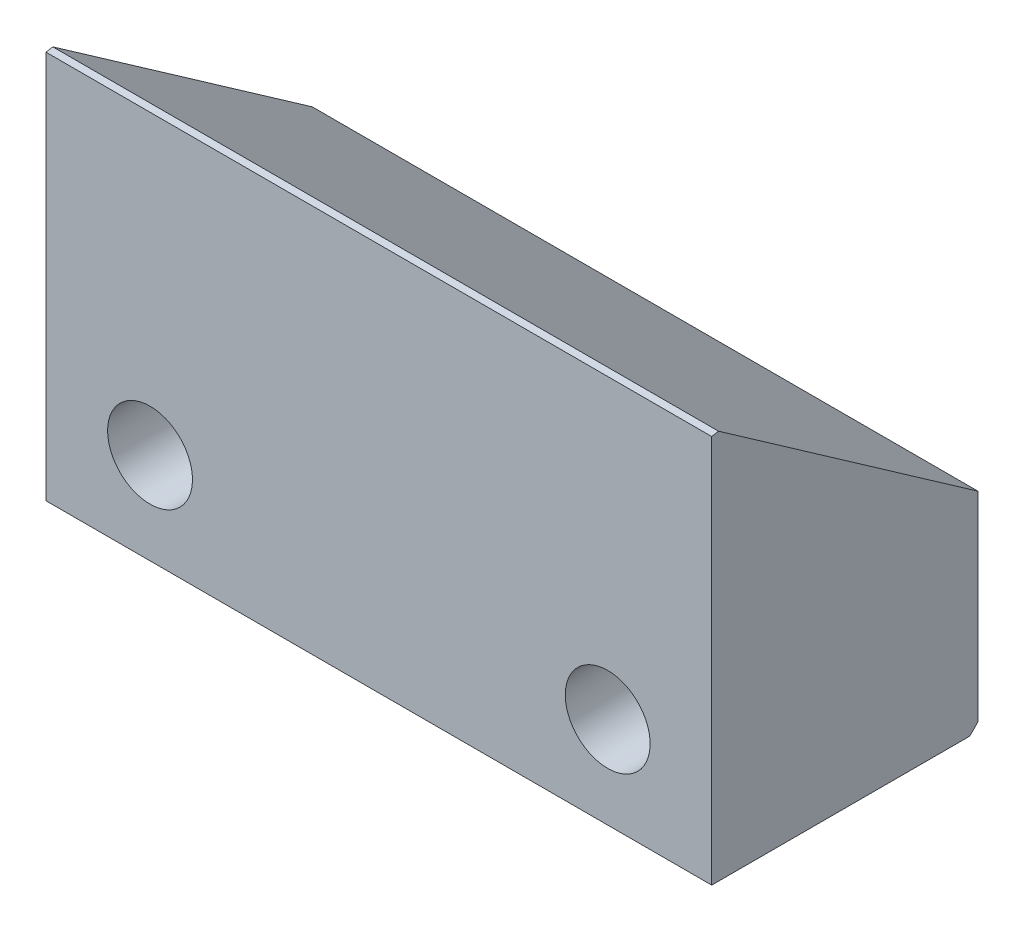
SolidWorks part; units mm, degrees
ref_plane "Front Plane" through (0, 0, 0) normal (0, 0, 1) x (1, 0, 0)
ref_plane "Top Plane" through (0, 0, 0) normal (0, 1, 0) x (1, 0, 0)
ref_plane "Right Plane" through (0, 0, 0) normal (1, 0, 0) x (0, 0, -1)
other "Configuration Table"
sketch "Sketch1" plane through (0, 0, 0) normal (1, 0, 0) x (0, 0, -1)
  line L0 (0, 0) -> (0, 47.4066)
  line L1 (0, 47.4066) -> (32, 25)
  line L2 (32, 25) -> (32, 0)
  line L3 (32, 0) -> (0, 0)
  dimension "D1" = 55
  dimension "D2" = 25
  dimension "D3" = 32
extrude "Boss-Extrude1" add sketch "Sketch1" along normal blind 80
sketch "Sketch2" plane through (0, 0, -32) normal (0, 0, -1) x (-1, 0, 0)
  line L0 (-40, 0) -> (-40, 11) construction
  line L1 (-80, 0) -> (0, 0) construction
  line L2 (-40, 11) -> (-12.5, 11) construction
  point P5 (-12.5, 11)
  point P9 (-12.5, 11)
  dimension "D1" = 11
  dimension "D2" = 27.5
hole_wizard "M12 Tapped Hole1" positions "Sketch2" profile "Sketch3" tap size "M12" standard "GB"
sketch "Sketch3" plane through (12.5, 11, -32) normal (1, 0, 0) x (0, 1, 0)
  line L0 (0, 0) -> (0, 63.0644)
  line L1 (0, 63.0644) -> (5.1, 60)
  line L2 (5.1, 60) -> (5.1, 0.925)
  line L3 (5.1, 0.925) -> (6.025, 0)
  line L5 (6.025, 0) -> (0, 0)
  line L6 (-5.1, 0.925) -> (-6.025, 0) construction
  line L10 (0, 63.0644) -> (-5.1, 60) construction
  line L11 (0, -6.35) -> (0, 107.95) construction
  dimension "螺纹孔钻头直径" = 10.2
  dimension "螺纹孔钻头深度" = 60
  dimension "近端锥形沉头孔直径" = 12.05
  dimension "近端锥形沉头孔角度" = 90
  dimension "导头角度" = 118
cosmetic thread "Hole Thread1" parameters "D1"=24, "D2"=12
ref_plane "Plane1" through (40, 0, 0) normal (1, 0, 0) x (0, 0, -1)
mirror "Mirror1" about plane through (40, 0, 0) normal (1, 0, 0) of "M12 Tapped Hole1"
chamfer "Chamfer1" distance 1 angle 45 2 edges at (40, 0, -32) (40, 47.4066, 0)
